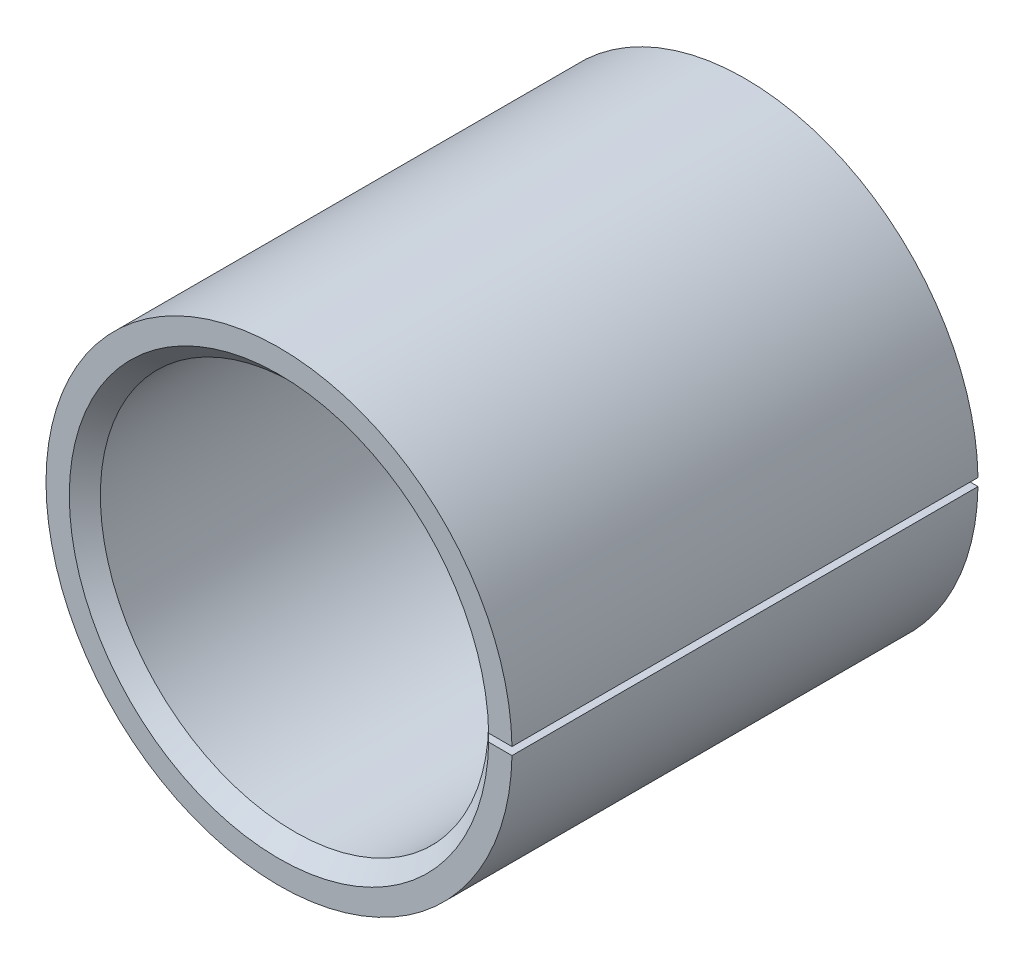
from build123d import *

# Parameters (mm, degrees)
SKETCH1_R           = 3
SKETCH1_R_2         = 2.5
BOSS_EXTRUDE1_DEPTH = 6
CHAMFER1_SIZE       = 0.2
SKETCH2_W           = 4.716397802
SKETCH2_H           = 0.1
CUT_EXTRUDE1_DEPTH  = 6


with BuildPart() as part:
    # Sketch1 → Boss-Extrude1 (new body)
    with BuildSketch(Plane.XY):
        Circle(SKETCH1_R)
        Circle(SKETCH1_R_2, mode=Mode.SUBTRACT)
    extrude(amount=BOSS_EXTRUDE1_DEPTH)

    # Chamfer1
    chamfer1_edges = [part.edges().sort_by_distance(p)[0] for p in [
        (-2.5, 0, 0),
        (-2.5, 0, 6),
    ]]
    chamfer(chamfer1_edges, length=CHAMFER1_SIZE)

    # Sketch2 → Cut-Extrude1 (cut)
    with BuildSketch(Plane.XY.offset(6)):
        with Locations((3, 0)):
            Rectangle(SKETCH2_W, SKETCH2_H)
    extrude(amount=-CUT_EXTRUDE1_DEPTH, mode=Mode.SUBTRACT)


solid = part.part
